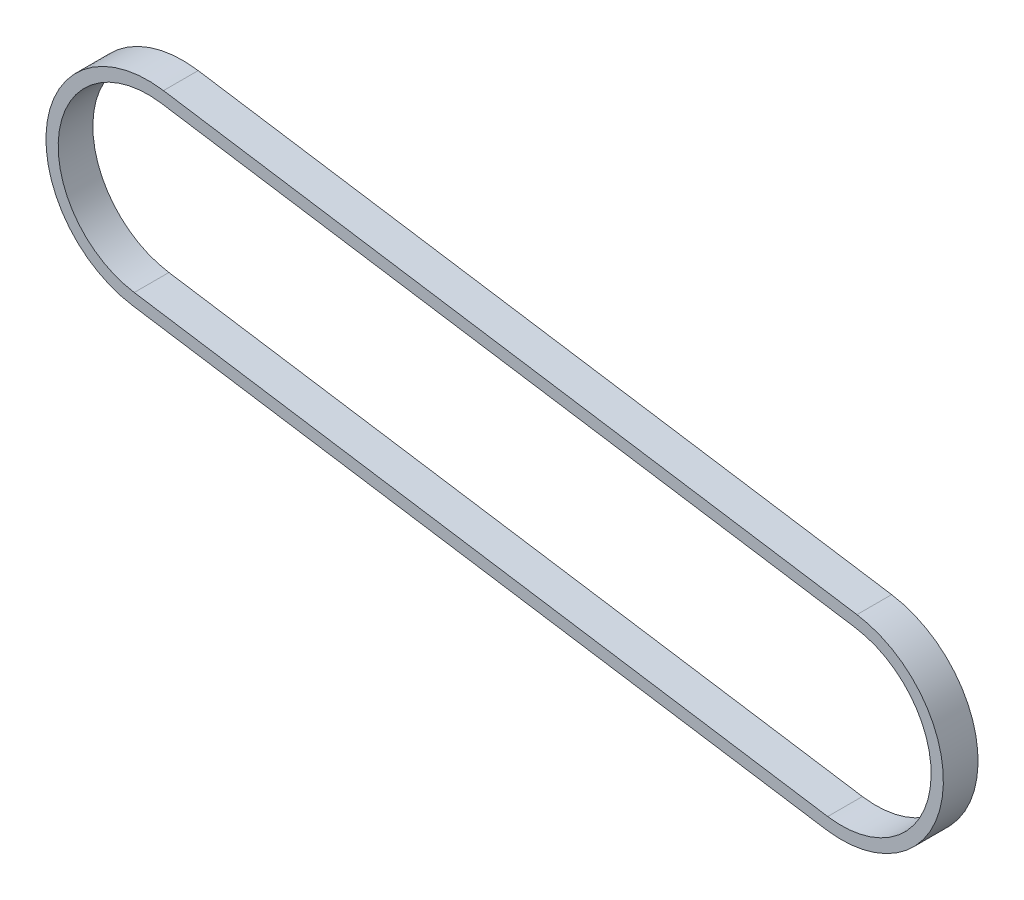
SolidWorks part; units mm, degrees
material "45+钨钢 "
ref_plane "Front Plane" through (0, 0, 0) normal (0, 0, 1) x (1, 0, 0)
ref_plane "Top Plane" through (0, 0, 0) normal (0, 1, 0) x (1, 0, 0)
ref_plane "Right Plane" through (0, 0, 0) normal (1, 0, 0) x (0, 0, -1)
sketch "Sketch2" plane through (0, 0, 0) normal (0, 0, 1) x (1, 0, 0)
  line L0 (0, 0) -> (1, 0) construction
  line L1 (0, 0) -> (0, 1) construction
  line L2 (7.6302, 49.4144) -> (347.6302, -3.0856)
  line L3 (332.3698, -101.9144) -> (-7.6302, -49.4144)
  arc A0 (-7.6302, -49.4144) -> (7.6302, 49.4144) centre (0, 0) cw
  arc A1 (347.6302, -3.0856) -> (332.3698, -101.9144) centre (340, -52.5) cw
extrude "Extrude-Thin1" add sketch "Sketch2" along normal mid plane 17 thin
